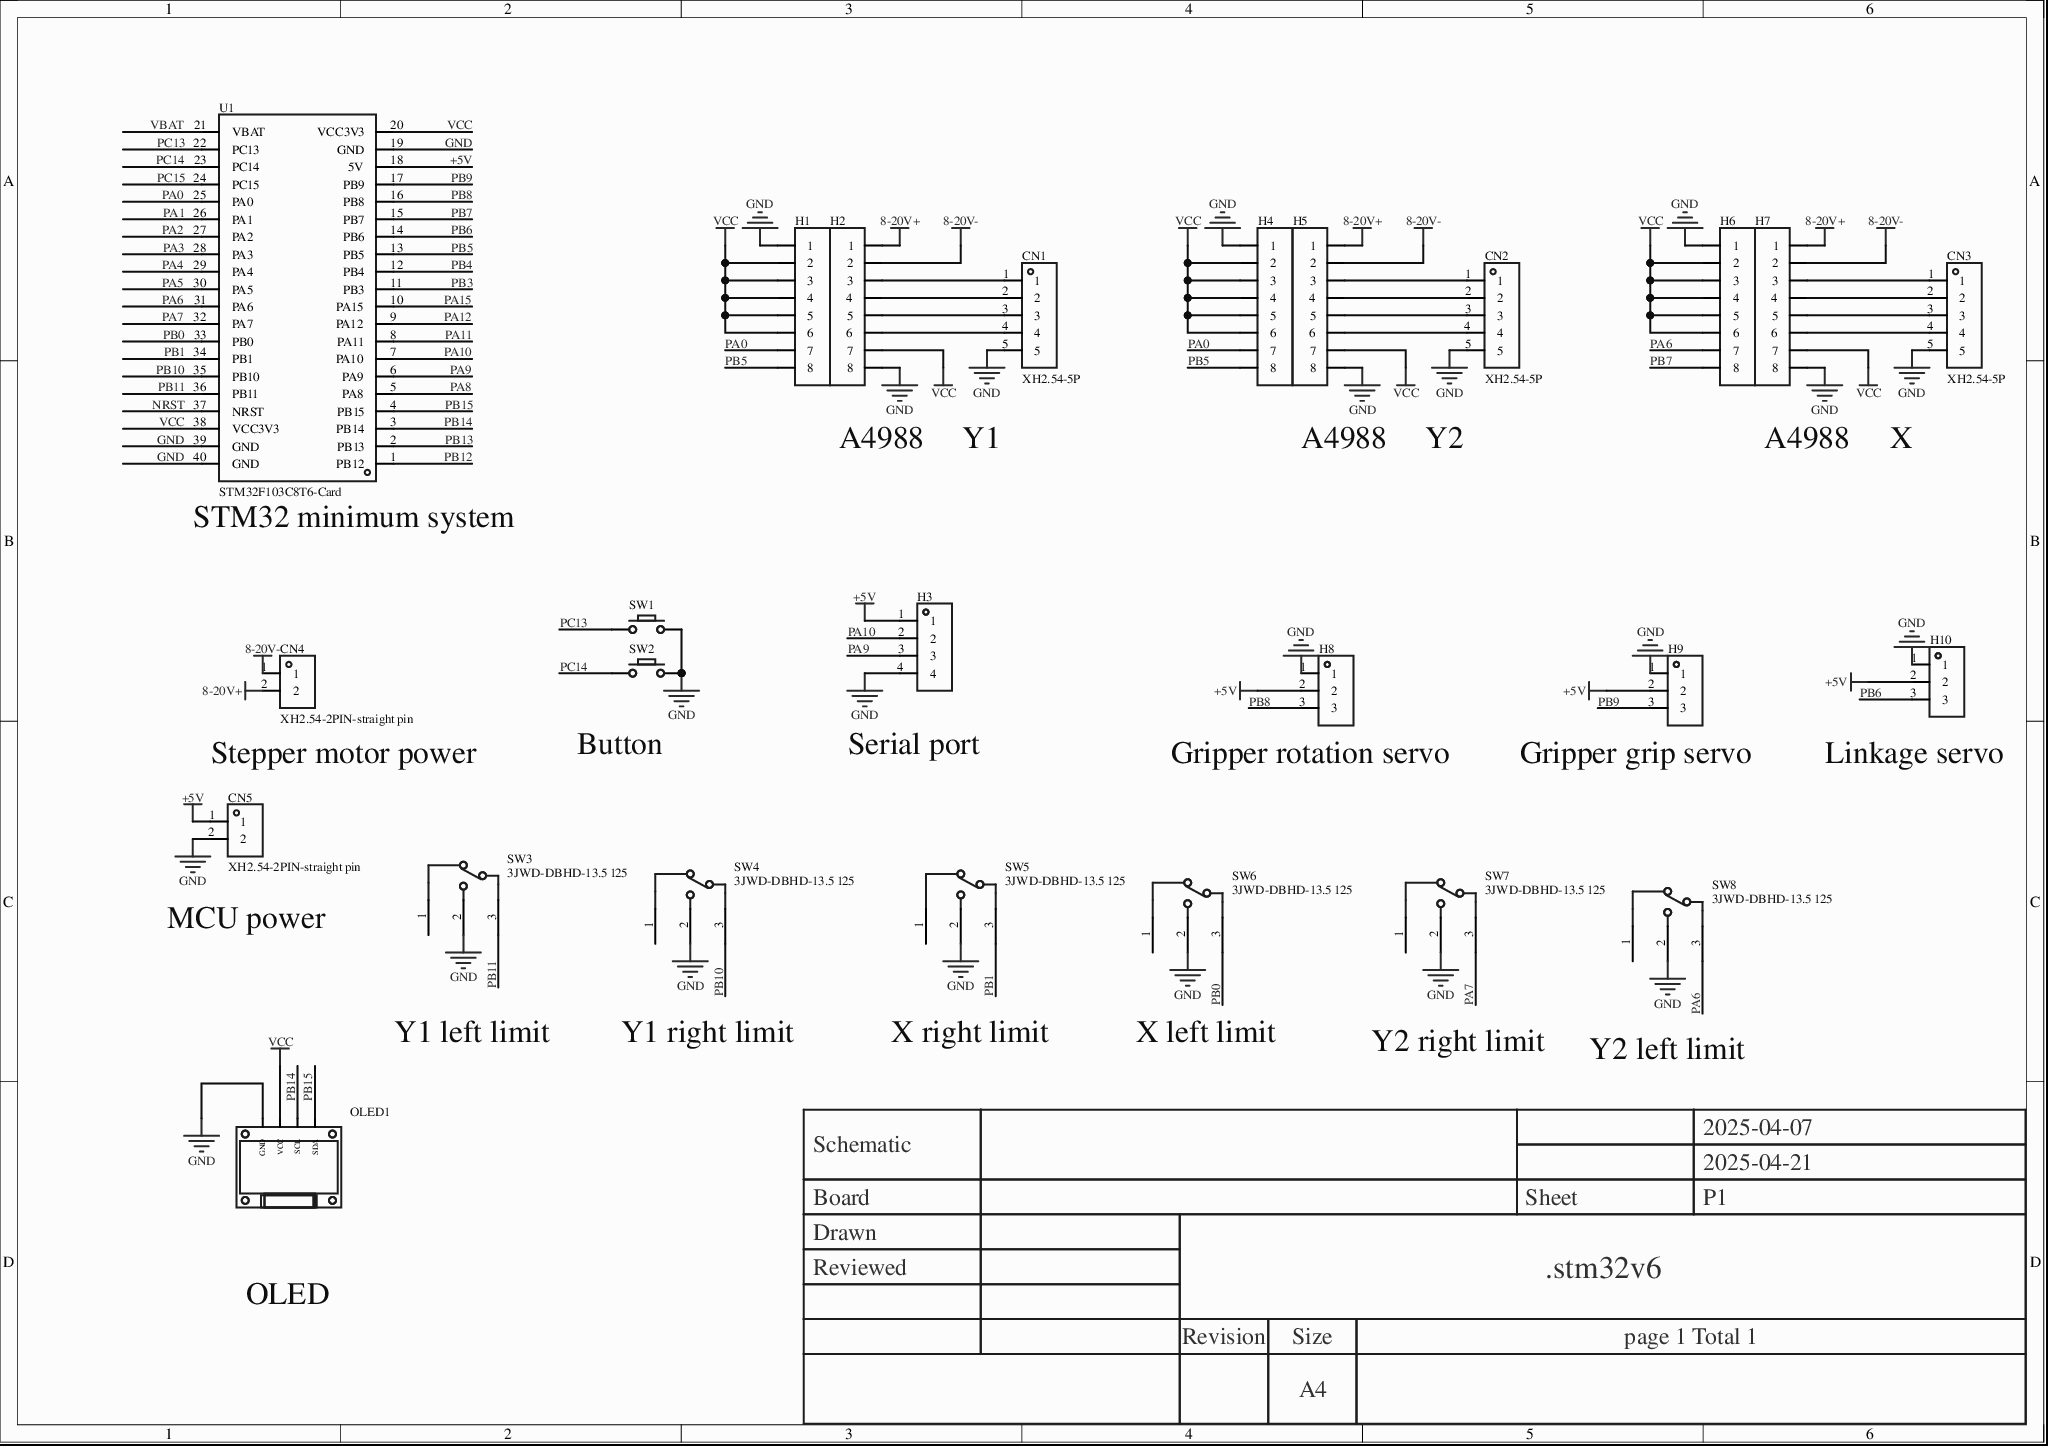
[diagram p0: MISC89043-3.schdoc]
# Altium project MISC89043-2.PrjPcb
1 sheet, 25 parts. Net scope: global (net labels, ports and power ports of the same name join across sheets).
Board file: MISC89043.pcbdoc

## Sheet MISC89043-3.schdoc
size 297 x 209 mm; Version: V1.0; @Project Name: MISC89043; @Page Count: 1; @Update Date: 2026-04-13; @Create Date: 2026-04-13; @Schematic Name: MISC89043; @Page No: 1; @Create Time: 23:22:16; @Update Time: 17:32:40; @Board Name: MISC89043

### Parts
CN1  XH2.54-5P  [CONN-TH_5P-P2.54_C9900008095]
CN2  XH2.54-5P  [CONN-TH_5P-P2.54_C9900008095]
CN3  XH2.54-5P  [CONN-TH_5P-P2.54_C9900008095]
CN4  XH2.54-2PIN-straight pin  [CONN-TH_XH2.54-2P]
CN5  XH2.54-2PIN-straight pin  [CONN-TH_XH2.54-2P]
H1  (no value)  [HDR-TH_8P-P2.54-V-F-1]
H2  (no value)  [HDR-TH_8P-P2.54-V-F-1]
H3  (no value)  [HDR-TH_4P-P2.54-V-F]
H4  (no value)  [HDR-TH_8P-P2.54-V-F-1]
H5  (no value)  [HDR-TH_8P-P2.54-V-F-1]
H6  (no value)  [HDR-TH_8P-P2.54-V-F-1]
H7  (no value)  [HDR-TH_8P-P2.54-V-F-1]
H8  (no value)  [HDR-TH_3P-P2.54-V-F]
H9  (no value)  [HDR-TH_3P-P2.54-V-F]
H10  (no value)  [HDR-TH_3P-P2.54-V-F]
OLED1  (no value)  [0.96OLED_4P]
SW1  (no value)  [Key_TH_3.5x6x4.3]
SW2  (no value)  [Key_TH_3.5x6x4.3]
SW3  3JWD-DBHD-13.5 125  [SW-TH_SHOU-HAN_3JWD-DBHD-13.5]
SW4  3JWD-DBHD-13.5 125  [SW-TH_SHOU-HAN_3JWD-DBHD-13.5]
SW5  3JWD-DBHD-13.5 125  [SW-TH_SHOU-HAN_3JWD-DBHD-13.5]
SW6  3JWD-DBHD-13.5 125  [SW-TH_SHOU-HAN_3JWD-DBHD-13.5]
SW7  3JWD-DBHD-13.5 125  [SW-TH_SHOU-HAN_3JWD-DBHD-13.5]
SW8  3JWD-DBHD-13.5 125  [SW-TH_SHOU-HAN_3JWD-DBHD-13.5]
U1  STM32F103C8T6-Card  [CONN-TH_L53.3-W22.9_STM32F103C8T6-CARD]

### Nets
8-20V+: CN4.2 H2.1 H5.1 H7.1
8-20V-: CN4.1 H2.2 H5.2 H7.2
+5V: CN5.1 H3.1 H8.2 H9.2 H10.2 U1.18(5V)
GND: CN1.5 CN2.5 CN3.5 CN5.2 H1.1 H2.8 H3.4 H4.1 H5.8 H6.1 H7.8 H8.1 H9.1 H10.1 OLED1.1(GND) SW1.B SW2.B SW3.2(ON) SW4.2(ON) SW5.2(ON) SW6.2(ON) SW7.2(ON) SW8.2(ON) U1.19(GND) U1.39(GND) U1.40(GND)
VCC: H1.2 H1.3 H1.4 H1.5 H1.6 H2.7 H4.2 H4.3 H4.4 H4.5 H4.6 H5.7 H6.2 H6.3 H6.4 H6.5 H6.6 H7.7 OLED1.2(VCC) U1.20(VCC3V3) U1.38(VCC3V3)
NRST: U1.37(NRST)
PA0: H1.7 H4.7 U1.25(PA0)
PA1: U1.26(PA1)
PA2: U1.27(PA2)
PA3: U1.28(PA3)
PA4: U1.29(PA4)
PA5: U1.30(PA5)
PA6: H6.7 SW8.3(NC) U1.31(PA6)
PA7: SW7.3(NC) U1.32(PA7)
PA8: U1.5(PA8)
PA9: H3.3 U1.6(PA9)
PA10: H3.2 U1.7(PA10)
PA11: U1.8(PA11)
PA12: U1.9(PA12)
PA15: U1.10(PA15)
PB0: SW6.3(NC) U1.33(PB0)
PB1: SW5.3(NC) U1.34(PB1)
PB3: U1.11(PB3)
PB4: U1.12(PB4)
PB5: H1.8 H4.8 U1.13(PB5)
PB6: H10.3 U1.14(PB6)
PB7: H6.8 U1.15(PB7)
PB8: H8.3 U1.16(PB8)
PB9: H9.3 U1.17(PB9)
PB10: SW4.3(NC) U1.35(PB10)
PB11: SW3.3(NC) U1.36(PB11)
PB12: U1.1(PB12)
PB13: U1.2(PB13)
PB14: OLED1.3(SCL) U1.3(PB14)
PB15: OLED1.4(SDA) U1.4(PB15)
PC13: SW1.A U1.22(PC13)
PC14: SW2.A U1.23(PC14)
PC15: U1.24(PC15)
VBAT: U1.21(VBAT)
NetCN1_1: CN1.1 H2.3
NetCN1_2: CN1.2 H2.4
NetCN1_3: CN1.3 H2.5
NetCN1_4: CN1.4 H2.6
NetCN2_1: CN2.1 H5.3
NetCN2_2: CN2.2 H5.4
NetCN2_3: CN2.3 H5.5
NetCN2_4: CN2.4 H5.6
NetCN3_1: CN3.1 H7.3
NetCN3_2: CN3.2 H7.4
NetCN3_3: CN3.3 H7.5
NetCN3_4: CN3.4 H7.6

Not connected (* = marked no-connect by the designer): SW3 1(C); SW4 1(C); SW5 1(C); SW6 1(C); SW7 1(C); SW8 1(C)

### Notes on the sheet
- A4988     Y1
- A4988     Y2
- A4988     X
- (near U1) STM32 minimum system
- Stepper motor power
- (near SW2) Button
- (near H3) Serial port
- (near H8) Gripper rotation servo
- (near H9) Gripper grip servo
- (near H10) Linkage servo
- (near CN5) MCU power
- Y1 left limit
- Y1 right limit
- X right limit
- X left limit
- Y2 right limit
- Y2 left limit
- OLED
- 2025-04-07
- Schematic
- Board
- Sheet
- 2025-04-21
- P1
- Drawn
- Reviewed
- .stm32v6
- Revision
- Size
- A4
- page 1 Total 1

### Library data of the parts
CN1-CN3 = XH2.54-5P: Symbol: XH2.54-5P_C9900017328; AddInBom: yes; ModelId: 432b56fff78447668e00d44b84af482c0819f05c4eef4c71ace90d822a990e87; ModelTransform: 590.55,224.41294,0,0,0,0,0,-21.654,-118.11; Device: XH2.54-5P; LCSC Part Name: XH2.54-5P; SupplierPart: C9900017328; ManufacturerPart: XH2.54-5P; Supplier Footprint: XH2.54-5P; JLCPCB Part Class: Extended Part; Supplier: LCSC; ConvertToPcb: yes; FootprintName: CONN-TH_5P-P2.54_C9900008095; ModelName: CONN-TH_5P-P2.54_C9900008095
CN4 CN5 = XH2.54-2PIN-直针: AddInBom: yes; ModelId: c3cc11bd8b8748c1ae6bc231aac3a1ff0819f05c4eef4c71ace90d822a990e87; ModelTransform: 296.889,230.315,0,0,0,0,0,26.653,-137.795; Symbol: XH2.54-2PIN-straight pin; Device: XH2.54-2PIN-straight pin; LCSC Part Name: XH2.54-2PIN-直针; SupplierPart: C9900011425; ManufacturerPart: XH2.54-2PIN-直针; Supplier Footprint: XH2.54-2PIN; JLCPCB Part Class: Extended Part; Supplier: LCSC; ConvertToPcb: yes; FootprintName: CONN-TH_XH2.54-2P; ModelName: CONN-TH_XH2.54-2P
H1 H2 H4-H7 = HDR-F_2.54_1x8P: Symbol: Header-Female-2.54_1x8; AddInBom: yes; ModelId: 0f7e4d9227ef4fa08d5469c22cc70cdb; ModelName: HDR-F-2.54_1x8; ModelTransform: 799.99844,100,0,0,0,0,0,0,-118.11; Device: HDR-F_2.54_1x8P; ConvertToPcb: yes; FootprintName: HDR-TH_8P-P2.54-V-F-1; SupplierPart: C27438; Supplier Footprint: 插件
H3 = HDR-F_2.54_1x4P: Symbol: 2.54-1*4P female; 3D Model: d187812051054f85879fcaa51a310d8e0819f05c4eef4c71ace90d822a990e87; 3D Model Transform: 419.6842,98.464,0,0,0,0,0,0,-118.11; ConvertToPcb: yes; Device: HDR-F_2.54_1x4P; Supplier Part: C2718488; Supplier Footprint: 插件; AddInBom: yes; FootprintName: HDR-TH_4P-P2.54-V-F; ModelName: HDR-TH_4P-P2.54-V-F
H8-H10 = HDR-F_2.54_1x3P: Symbol: PM254V-11-03-H85; ConvertToPcb: yes; ModelId: f3b3cc5aae9641bf9e56fc160cef875b; ModelName: HDR2.54-F-LI-1X3P; ModelTransform: 299.9994,100,0,0,0,0,0,0,-118.11; Device: HDR-F_2.54_1x3P; AddInBom: yes; SupplierPart: C541850; Supplier Footprint: 插件; FootprintName: HDR-TH_3P-P2.54-V-F
OLED1 = 0.96OLED模块_4P: Device: 0.96OLED module_4P; ConvertToPcb: yes; ModelId: 79c000fdb68d45a296c2e9bedf4f9055; ModelTransform: 1393.69792,1318.895,0,0,0,0,0,-560.079,-137.795; Symbol: 0.96OLED module_4P; FootprintName: 0.96OLED_4P; AddInBom: yes; Supplier Footprint: 插件; ModelName: 0.96OLED_4P
SW1 SW2 = Key_TH_3.5x6x4.3: 3D Model: c3523f9014d949d7ba5445190a3178990819f05c4eef4c71ace90d822a990e87; 3D Model Transform: 308.49,137.8,335.08,0,0,0,0,0,-129.92; ConvertToPcb: yes; ModelName: SW-TH_L6.0-W3.5-H5.0-P6.5; Symbol: Key_TH_3.5x6x4.3; Device: Key_TH_3.5x6x4.3; Supplier Footprint: 插件; AddInBom: yes; FootprintName: Key_TH_3.5x6x4.3
SW3-SW8 = 3JWD-DBHD-13.5 125: Circuit structure: SPDT; rated current (DC): 50mA; rated voltage (DC): 125V; rated current (AC): -; rated voltage (AC): -; operating life: 5万 cycles;; Manufacturer: SHOU HAN(首韩); AddInBom: yes; ModelId: a958994ff2844270919ff0f2ba7a126e0819f05c4eef4c71ace90d822a990e87; ModelTransform: 564.511,224.409,0,0,0,0,29.528,0,-118.11; Switch Height: 6.6mm; Symbol: 3JWD-DBHD-13.5 125; Device: 3JWD-DBHD-13.5 125; LCSC Part Name: 鼠标3脚微动 红点直柄13.5; SupplierPart: C2906291; ManufacturerPart: 3JWD-DBHD-13.5 125; Supplier Footprint: 插件,12.8x5.7mm; JLCPCB Part Class: Extended Part; Datasheet: https://example.com/datasheet/3JWD-DBHD-13.5%2520125/3179001.html; Supplier: LCSC; ConvertToPcb: yes; FootprintName: SW-TH_SHOU-HAN_3JWD-DBHD-13.5; ModelName: SW-TH_SHOU-HAN_3JWD-DBHD-13.5; Circuit: SPDT; Actuator Style: -; Length: 12.8mm; Width: 5.8mm; Current Rating (DC): 50mA; Voltage Rating (DC): 125V; Current Rating (AC): -; Voltage Rating (AC): -; Life: 5万 cycles; Termination Style: PCB pins; Operating Temperature: -25℃~+85℃; Operating Height: -
U1 = STM32F103C8T6-Card: AddInBom: yes; Device: STM32F103C8T6-Card; Symbol: STM32F103C8T6-CARD; FootprintName: CONN-TH_L53.3-W22.9_STM32F103C8T6-CARD; LCSC Part Name: STM32F103C8T6-Card; SupplierPart: C9900077949; ManufacturerPart: STM32F103C8T6-Card; Supplier Footprint: 插件; Supplier: LCSC; ConvertToPcb: yes